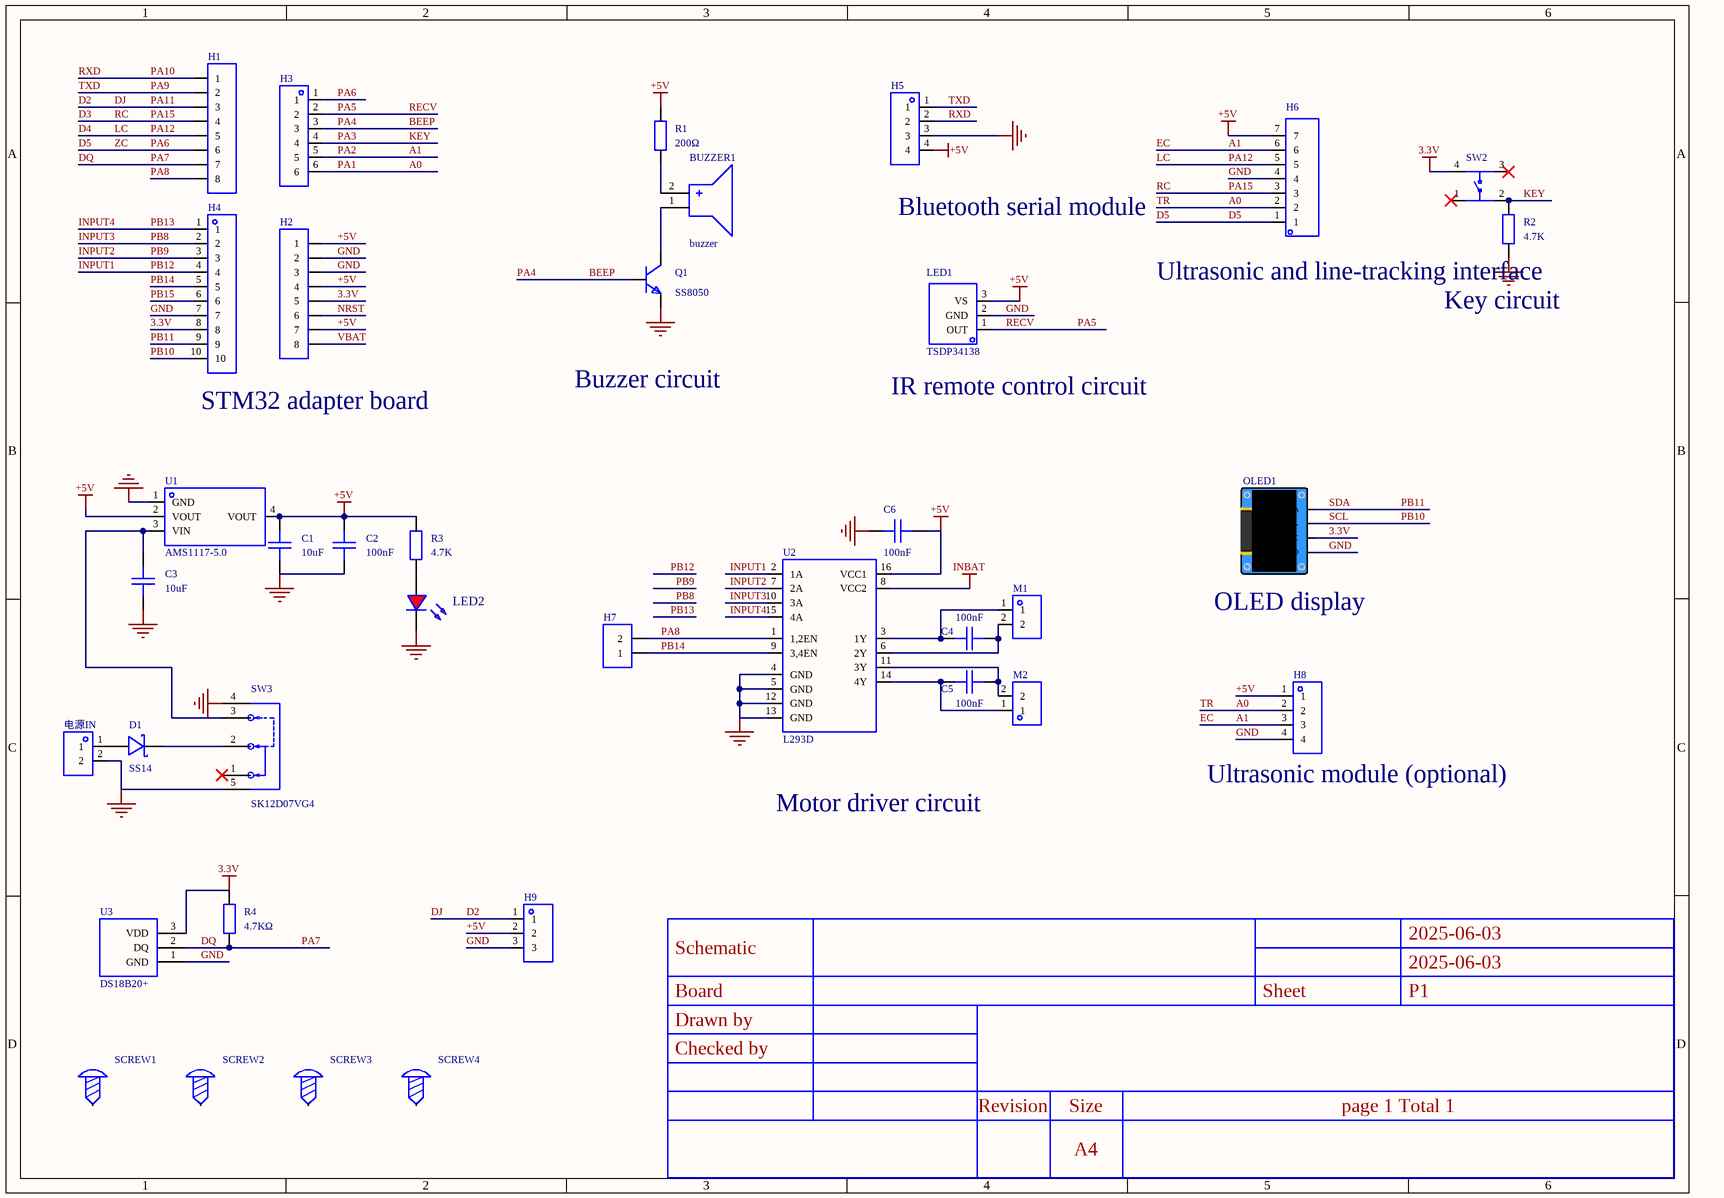
[diagram p0: MISC61257-3.schdoc]
# Altium project MISC61257-2.PrjPcb
1 sheet, 37 parts. Net scope: global (net labels, ports and power ports of the same name join across sheets).
Board file: MISC61257.pcbdoc

## Sheet MISC61257-3.schdoc
size 297 x 209 mm; Version: V1.0; @Project Name: MISC61257; @Page Count: 1; @Update Date: 2025-06-03; @Create Date: 2025-06-03; @Schematic Name: MISC61257; @Page No: 1; @Create Time: 12:58:07; @Update Time: 16:45:28; @Board Name: MISC61257

### Parts
BUZZER1  buzzer  [BUZ-TH_BD12.0-P6.00-D0.9-RD]
C1  10uF  [C0805]
C2  100nF  [C0805]
C3  10uF  [C0805]
C4  100nF  [C0805]
C5  100nF  [C0805]
C6  100nF  [C0805]
D1  SS14  [SMA_L4.2-W2.6-LS5.3-RD]
H1  (no value)  [HDR-TH_8P-P2.54-V-F-1]
H2  (no value)  [HDR-TH_8P-P2.54-V-F-1]
H3  (no value)  [HDR-TH_6P-P2.54-V-F]
H4  (no value)  [HDR-TH_10P-P2.54-V-F]
H5  (no value)  [HDR-TH_4P-P2.54-V-F]
H6  (no value)  [HDR-TH_7P-P2.54-V-F]
H7  (no value)  [HDR-TH_2P-P2.54-V-F]
H8  (no value)  [HDR-TH_4P-P2.54-V-F]
H9  (no value)  [HDR-TH_3P-P2.54-V-M]
LED1  TSDP34138  [SENSOR-TH_TSDP34138]
LED2  (no value)  [LED_0603]
M1  HX25003-2A  [CONN-TH_2P-P2.50_HX25003-2A]  (value not drawn)
M2  HX25003-2A_C2915012  [CONN-TH_2P-P2.50_HX25003-2A]  (value not drawn)
OLED1  (no value)  [0.96OLED_4P]
Q1  SS8050  [SOT-23-3_L2.9-W1.3-P1.90-LS2.4-BR]
R1  200Ω  [R0805]
R2  4.7K  [R0805]
R3  4.7K  [R0805]
R4  4.7KΩ  [R0805]
SCREW1  (no value)  [M3螺丝]
SCREW2  (no value)  [M3螺丝]
SCREW3  (no value)  [M3螺丝]
SCREW4  (no value)  [M3螺丝]
SW2  TS1702-CZ65HBS  [SW-TH_4P-L6.0-W6.0-P4.50-LS6.3]  (value not drawn)
SW3  SK12D07VG4  [SW-TH_SK12D07VG4]
U1  AMS1117-5.0  [SOT-223_L6.5-W3.5-P2.30-LS7.0-BR]
U2  L293D  [DIP-16_L20.0-W6.4-P2.54-LS7.6-BL]
U3  DS18B20+  [TO-92-3_L4.9-W3.7-P1.27-L]
电源IN  HX25003-2A  [CONN-TH_2P-P2.50_HX25003-2A]  (value not drawn)

### Nets
3.3V: H2.5 H4.8 OLED1.2(VCC) R4.2 SW2.4 U3.3(VDD)
+5V: C1.2 C2.2 C6.2 H2.1 H2.4 H2.7 H5.4 H6.7 H8.1 H9.2 LED1.3(VS) R1.2 R3.2 U1.2(VOUT) U1.4(VOUT) U2.16(VCC1)
GND: C1.1 C2.1 C3.1 C6.1 H2.2 H2.3 H4.7 H5.3 H6.4 H8.4 H9.3 LED1.2(GND) LED2.1(C) OLED1.1(GND) Q1.2(E) R2.1 SW3.4 SW3.5 U1.1(GND) U2.4(GND) U2.5(GND) U2.12(GND) U2.13(GND) U3.1(GND) 电源IN.2
INBAT: U2.8(VCC2)
A0: H3.6 H6.2 H8.2  [also labelled PA1, TR]
A1: H3.5 H6.6 H8.3  [also labelled EC, PA2]
BEEP: H3.3 Q1.1(B)  [also labelled PA4]
D2: H1.3 H9.1  [also labelled DJ, PA11]
D3: H1.4 H6.3  [also labelled PA15, RC]
D4: H1.5 H6.5  [also labelled LC, PA12]
D5: H1.6 H3.1 H6.1  [also labelled PA6, ZC]
DQ: H1.7 R4.1 U3.2(DQ)  [also labelled PA7]
INPUT1: H4.4 U2.2(1A)  [also labelled PB12]
INPUT2: H4.3 U2.7(2A)  [also labelled PB9]
INPUT3: H4.2 U2.10(3A)  [also labelled PB8]
INPUT4: H4.1 U2.15(4A)  [also labelled PB13]
KEY: H3.4 R2.2 SW2.2  [also labelled PA3]
NRST: H2.6
PA5: H3.2 LED1.1(OUT)  [also labelled RECV]
PA8: H1.8 H7.2 U2.1(1,2EN)
PA9: H1.2 H5.1  [also labelled TXD]
PA10: H1.1 H5.2  [also labelled RXD]
PB10: H4.10 OLED1.3(SCL)  [also labelled SCL]
PB11: H4.9 OLED1.4(SDA)  [also labelled SDA]
PB14: H4.5 H7.1 U2.9(3,4EN)
PB15: H4.6
VBAT: H2.8
NetBUZZER1_1: BUZZER1.1(-) Q1.3(C)
NetBUZZER1_2: BUZZER1.2(+) R1.1
NetC3_2: C3.2 SW3.3 U1.3(VIN)
NetC4_1: C4.1 M1.1 U2.3(1Y)
NetC4_2: C4.2 M1.2 U2.6(2Y)
NetC5_1: C5.1 M2.1 U2.14(4Y)
NetC5_2: C5.2 M2.2 U2.11(3Y)
NetD1_1: D1.1(K) SW3.2
NetD1_2: D1.2(A) 电源IN.1
NetLED2_2: LED2.2(A) R3.1

Not connected (* = marked no-connect by the designer): SCREW1 1; SCREW2 1; SCREW3 1; SCREW4 1; SW2 1* 3*; SW3 1*

### Notes on the sheet
- (near H5) Bluetooth serial module
- (near R2) Ultrasonic and line-tracking interface
- (near R2) Key circuit
- STM32 adapter board
- Buzzer circuit
- (near LED1) IR remote control circuit
- (near OLED1) OLED display
- (near H8) Ultrasonic module (optional)
- Motor driver circuit
- 2025-06-03
- Schematic
- Board
- Sheet
- P1
- Drawn by
- Checked by
- Revision
- Size
- A4
- page 1 Total 1

### Library data of the parts
BUZZER1 = buzzer: AddInBom: yes; ModelId: af17e4151ed84fc2a628230bf2376363; ModelTransform: 472.44,472.176,0,270,0,0,0,0,-196.85; Symbol: BUZZER; Device: buzzer; LCSC Part Name: buzzer; SupplierPart: C9900014030; ManufacturerPart: buzzer; Supplier Footprint: buzzer; JLCPCB Part Class: Extended library; Supplier: LCSC; ConvertToPcb: yes; FootprintName: BUZ-TH_BD12.0-P6.00-D0.9-RD; ModelName: BUZ-TH_BD12.0-P6.00-D0.9-RD
C1-C6 = CAP_0805: ConvertToPcb: yes; SymbolName: CapAcitance; ModelId: 1ba041120af144c991958decab20d241; ModelName: C0805_L2.0-W1.3-H1.3; ModelTransform: 78.74,51.181,0,0,0,0,0,0.0005,0; Device: CAP_0805; AddInBom: yes; Supplier Footprint: 0805; FootprintName: C0805
  C1 C3: Value: 10uF
  C2 C4-C6: Value: 100nF
D1 = SS14_C2480: Diode configuration: single; forward voltage (Vf): 550mV@1A; DC reverse voltage (Vr): 40V; rectifier current: 1A;; Manufacturer: MDD(辰达半导体); AddInBom: yes; ModelId: c9e8185d46a94015b9fa58a531b156cf; ModelTransform: 204.83943,103.346,0,0,0,0,-0.001,0.001,0; Reverse Leakage Current (Ir): 300uA@40V; Symbol: SS14; Device: SS14_C2480; LCSC Part Name: 电压:40V 电流:1A; SupplierPart: C2480; ManufacturerPart: SS14; Supplier Footprint: SMA(DO-214AC); Datasheet: https://atta.szlcsc.com/upload/public/pdf/source/20241121/B157EB417161760A7ED23035C0FAAB28.pdf; Supplier: LCSC; ConvertToPcb: yes; FootprintName: SMA_L4.2-W2.6-LS5.3-RD; ModelName: SMA_L4.2-W2.6-LS5.3-RD; Diode Configuration: Single; Voltage - Forward(Vf@If): 550mV@1A; Voltage - DC Reverse(Vr): 40V; Current - Rectified: 1A
H1 H2 = HDR-F_2.54_1x8P: Symbol: Header-Female-2.54_1x8; AddInBom: yes; ModelId: 0f7e4d9227ef4fa08d5469c22cc70cdb; ModelName: HDR-F-2.54_1x8; ModelTransform: 799.99844,100,0,0,0,0,0,0,-118.11; Device: HDR-F_2.54_1x8P; ConvertToPcb: yes; FootprintName: HDR-TH_8P-P2.54-V-F-1; SupplierPart: C27438; Supplier Footprint: 插件
H3 = HDR-F_2.54_1x6P: Symbol: Header-Female-2.54_1x6; ConvertToPcb: yes; ModelId: 0f5bcf94dcda47d085f24cdca1696fe9; ModelTransform: 619.684,94.488,0,0,0,0,0,0,-125.984; Device: HDR-F_2.54_1x6P; AddInBom: yes; SupplierPart: C40877; Supplier Footprint: 插件; FootprintName: HDR-TH_6P-P2.54-V-F; ModelName: HDR-TH_6P-P2.54-V-F
H4 = HDR-F_2.54_1x10P: Symbol: X5511FV-10-C70D30-1000; AddInBom: yes; ModelId: 08a5ee31ec6747838a696d2ac093ffa4; ModelName: HDR-TH_10P-P2.54-F-LI-1X10P; ModelTransform: 1009.87987,100,0,0,0,0,0,0,-125.984; Device: HDR-F_2.54_1x10P; ConvertToPcb: yes; FootprintName: HDR-TH_10P-P2.54-V-F; SupplierPart: C2684744; Supplier Footprint: 插件
H5 H8 = HDR-F_2.54_1x4P: Symbol: 2.54-1*4P female; ConvertToPcb: yes; ModelId: d187812051054f85879fcaa51a310d8e; ModelTransform: 419.6842,98.464,0,0,0,0,0,0,-118.11; Device: HDR-F_2.54_1x4P; AddInBom: yes; SupplierPart: C2718488; Supplier Footprint: 插件; FootprintName: HDR-TH_4P-P2.54-V-F; ModelName: HDR-TH_4P-P2.54-V-F
H6 = HDR-F_2.54_1x7P: Symbol: 220S-1*7P H=8.5MM Ytype Gold-plated; ConvertToPcb: yes; ModelId: 4c31987253bc43b9b52c17be2a6d3f91; ModelName: HDR-TH_7P-P2.54-F-LI-1X7P; ModelTransform: 715.7466,94.488,0,0,0,0,0,0,-118.11; Device: HDR-F_2.54_1x7P; AddInBom: yes; SupplierPart: C124418; Supplier Footprint: 插件; FootprintName: HDR-TH_7P-P2.54-V-F
H7 = HDR-F_2.54_1x2P: Symbol: Header-Female-2.54_1x2; ConvertToPcb: yes; ModelId: a9450ef445564560a104363b9aacde4e; ModelName: HDR-TH_2P-P2.54-F-LI-1X2P; ModelTransform: 215.7476,98.425,0,0,0,0,0,0,-129.921; Device: HDR-F_2.54_1x2P; AddInBom: yes; SupplierPart: C49661; Supplier Footprint: 插件; FootprintName: HDR-TH_2P-P2.54-V-F
H9 = HDR-M_2.54_1x3P: Symbol: PZ254V-11-03P_C2937625; ConvertToPcb: yes; ModelId: bb473b6d38ff42a99216a4fcdbdcc4cb; ModelName: HDR-TH_3P-P2.54-M-LI-1X3P; ModelTransform: 299.9994,100,0,0,0,0,0,0,-118.11; Device: HDR-M_2.54_1x3P; AddInBom: yes; SupplierPart: C2937625; Supplier Footprint: 插件; FootprintName: HDR-TH_3P-P2.54-V-M
LED1 = TSDP34138: Operating voltage: 2.5V~5.5V; operating current: 350uA; receiving distance: 35m; centre frequency: 38.4kHz; receiving angle: ±45°;; Manufacturer: VISHAY(威世); AddInBom: yes; ModelId: 6b586f424e564dcfbb63032662918b0f; ModelTransform: 236.22,252.109,0,0,0,0,0,-80.709,-137.795; Power Consumption: 10mW; Symbol: TSDP34138; Device: TSDP34138; LCSC Part Name: 接收距离35m ±45°; SupplierPart: C143726; ManufacturerPart: TSDP34138; Supplier Footprint: SIP-3-2.54mm; JLCPCB Part Class: Extended library; Datasheet: https://atta.szlcsc.com/upload/public/pdf/source/20171128/C143726_15118626746271147266.pdf; Supplier: LCSC; ConvertToPcb: yes; FootprintName: SENSOR-TH_TSDP34138; ModelName: SENSOR-TH_TSDP34138; Supply Voltage: 2.5V~5.5V; Supply Current: 350uA; Transmission Distance: 35m; Center Frequency: 38.4kHz; Half Angle: ±45°; Operating Temperature: -25℃~+85℃
LED2 = LED_0603-R: Symbol: LED_R; Convert to PCB: yes; 3D Model: dd8257b0d61a4cd7b68939a056e08095; 3D Model Transform: 58.72,29.4,22.03,0,0,0,0,0,0; ModelName: LED-0603_R; Device: LED_0603-R; Add into BOM: yes; Supplier Footprint: 0603; FootprintName: LED_0603
M1 M2 电源IN = HX25003-2A_C2915012: AddInBom: yes; ModelId: 17c7be61cc0b4bc5acccb67e71c47088; ModelTransform: 295.275,232.283,0,180,0,0,0,-21.654,-129.921; Symbol: HX25003-2A_C2915012; Device: HX25003-2A_C2915012; LCSC Part Name: HX25003-2A; SupplierPart: C2915012; ManufacturerPart: HX25003-2A; Supplier Footprint: CONN-TH_2P-P2.50_HX25003-2A; JLCPCB Part Class: Extended library; Supplier: LCSC; ConvertToPcb: yes; FootprintName: CONN-TH_2P-P2.50_HX25003-2A; ModelName: CONN-TH_2P-P2.50_HX25003-2A
OLED1 = 0.96OLED模块_4P: Device: 0.96OLED module_4P; ConvertToPcb: yes; ModelId: 79c000fdb68d45a296c2e9bedf4f9055; ModelTransform: 1393.69792,1318.895,0,0,0,0,0,-560.079,-137.795; AddInBom: yes; SymbolName: 0.96OLED module_4P; FootprintName: 0.96OLED_4P; Supplier Footprint: 插件; ModelName: 0.96OLED_4P
Q1 = SS8050: Manufacturer: Doeshare(德芯); Symbol: SS8050_C2931717; AddInBom: yes; ModelId: c62791f0466c4ae2a892c056b845b0ca; ModelName: SOT-23-3P_L2.9-W1.3-H1.0-LS2.4-P0.95; ModelTransform: 98.425,114.173,0,180,0,0,0.0005,-0.0005,0; Device: SS8050; LCSC Part Name: NPN 25V 1.5A 120-400 SOT-23; SupplierPart: C2931717; ManufacturerPart: SS8050; Supplier Footprint: SOT-23; Datasheet: https://atta.szlcsc.com/upload/public/pdf/source/20220106/99F9A3DFCBDD91265C711555CE6390BF.pdf; Supplier: LCSC; ConvertToPcb: yes; FootprintName: SOT-23-3_L2.9-W1.3-P1.90-LS2.4-BR
R1-R4 = Res_0805: ConvertToPcb: yes; SymbolName: Resistor; ModelId: 37a81e68749a4138bd2dfa6897b24b85; ModelName: R0805_L2.0-W1.3-H0.6; ModelTransform: 78.74,51.181,0,0,0,0,0,-0.0005,0; Device: Res_0805; AddInBom: yes; Supplier Footprint: 0805; FootprintName: R0805
  R1: Value: 200Ω
  R2 R3: Value: 4.7K
  R4: Value: 4.7KΩ
SCREW1-SCREW4 = M3螺丝: Device: M3 screw; ConvertToPcb: yes; SymbolName: Screw hole; AddInBom: yes; Supplier Footprint: 插件; FootprintName: M3 screw
SW2 = TS1702-CZ65HBS: 6*6*6.5 直插 260GF  轻触开关  电路结构:单刀单掷 按钮形状：圆形按钮 触点电流:50mA 额定电压（DC）:12V 安装方式:直插 绝缘电阻:100MΩ 作用力:260GF±30gf 6*6*6.5  260GF  轻触开关; Manufacturer: BXCONN(宝讯); AddInBom: yes; ModelId: f12d4fb4f8314a3f92db4aebb329b432; ModelTransform: 306.99781,236.22,0,0,0,0,0,0,-137.795; Symbol: TS1702-CZ65HBS; Device: TS1702-CZ65HBS; LCSC Part Name: 6*6*6.5 直插    轻触开关; SupplierPart: C36936602; ManufacturerPart: TS1702-CZ65HBS; Supplier Footprint: 插件-4P,6x6mm; Datasheet: https://atta.szlcsc.com/upload/public/pdf/source/20240731/66C3AB51E4A5A2D6C8ACA806E745630D.pdf; Supplier: LCSC; ConvertToPcb: yes; FootprintName: SW-TH_4P-L6.0-W6.0-P4.50-LS6.3; ModelName: SW-TH_4P-L6.0-W6.0-P4.50-LS6.3
SW3 = SK12D07VG4: Circuit: single pole double throw; mounting: -; rated current (DC): 500mA; rated voltage (DC): 50V; rated current (AC): -; rated voltage (AC): -; mechanical life: 5千 cycles;; Manufacturer: SHOU HAN(首韩); AddInBom: yes; ModelId: 773c51563d484e3a80810244c5d56a16; ModelName: SW-TH_L8.7-W4.4-H4.0-P2.0; ModelTransform: 338.582,279.527,0,0,0,0,0,-51.181,-125.984; Circuit: SPDT; Actuator Style: Rectangular post; Pin Style: PC pin; Switch Height: 8.8mm; Symbol: SK12D07VG4; Device: SK12D07VG4; LCSC Part Name: 3脚2档位 卧插 滑动开关; SupplierPart: C393937; ManufacturerPart: SK12D07VG4; Supplier Footprint: 插件; JLCPCB Part Class: Extended library; Datasheet: https://atta.szlcsc.com/upload/public/pdf/source/20190521/C393937_939FE26E571CC67D2D532E953108A1B0.pdf; Supplier: LCSC; ConvertToPcb: yes; FootprintName: SW-TH_SK12D07VG4; Mounting Style: -; Current Rating (DC): 500mA; Voltage Rating (DC): 50V; Current Rating (AC): -; Voltage Rating (AC): -; Mechanical Life: 5千 cycles; Operating Temperature: -
U1 = AMS1117-5.0_C6187: Output type: fixed; operating voltage: 12V; output voltage: 5V; output current: 1A; power supply ripple rejection (PSRR): -; output polarity: positive;; Manufacturer: AMS; AddInBom: yes; ModelId: 925194bf9823436183a3e0b978a8d076; ModelName: SOT-223-4P_L6.5-W3.5-H1.6-LS7.0-P2.30; ModelTransform: 279.89794,255.905,0,180,0,0,0.0005,0.0005,0; Voltage Dropout: 1.3V@(1A); Number of Outputs: 1; Symbol: AMS1117-5.0; Device: AMS1117-5.0_C6187; LCSC Part Name: 输入12V 输出5V 1A; SupplierPart: C6187; ManufacturerPart: AMS1117-5.0; Supplier Footprint: SOT-223; Datasheet: https://atta.szlcsc.com/upload/public/pdf/source/20230918/E4B716057EE82179D88E8A0894830D59.pdf; Supplier: LCSC; ConvertToPcb: yes; FootprintName: SOT-223_L6.5-W3.5-P2.30-LS7.0-BR; Output Type: Fixed; Voltage - Supply: 12V; Output Voltage: 5V; Output Current: 1A; Power Supply Rejection Ratio (PSRR): -; standby current: -; Noise: -; Features: Overcurrent protection (OCP); Operating Temperature: -; Output Configuration: Positive
U2 = L293D: Push-pull quad-channel driver with diodes; Manufacturer: ST(意法半导体); AddInBom: yes; ModelId: 6857a51368f0401381488830b088717c; ModelName: DIP-16_L20.0-W6.4-H3.5-LS7.62-P2.54; ModelTransform: 787.4,311.8104,0,0,0,0,0,0,-125.984; Symbol: L293D; Device: L293D; LCSC Part Name: 600mA 有刷直流电机驱动芯片 36V; SupplierPart: C12340; ManufacturerPart: L293D; Supplier Footprint: DIP-16; Datasheet: https://atta.szlcsc.com/upload/public/pdf/source/20140724/1457707157802.pdf; Supplier: LCSC; ConvertToPcb: yes; FootprintName: DIP-16_L20.0-W6.4-P2.54-LS7.6-BL
U3 = DS18B20+: 1-Wire digital thermometer with programmable resolution; high-accuracy temperature measurement with minimal wiring, ideal for multi-sensor measurement systems; Manufacturer: ADI(亚德诺)/MAXIM(美信); AddInBom: yes; ModelId: db569d051dcd4484acf2f9e50678fca3; ModelTransform: 180.7872,141.4455,0,0,0,0,0,22.677,-196.85; Supply Voltage: 3V~5.5V; Symbol: DS18B20+; Device: DS18B20+; LCSC Part Name: DS18B20; SupplierPart: C9753; ManufacturerPart: DS18B20+; Supplier Footprint: TO-92; JLCPCB Part Class: Extended library; Datasheet: https://atta.szlcsc.com/upload/public/pdf/source/20170713/C118507_1499918901893816791.pdf; Supplier: LCSC; ConvertToPcb: yes; FootprintName: TO-92-3_L4.9-W3.7-P1.27-L; ModelName: TO-92-3_L4.9-W3.7-P1.27-L